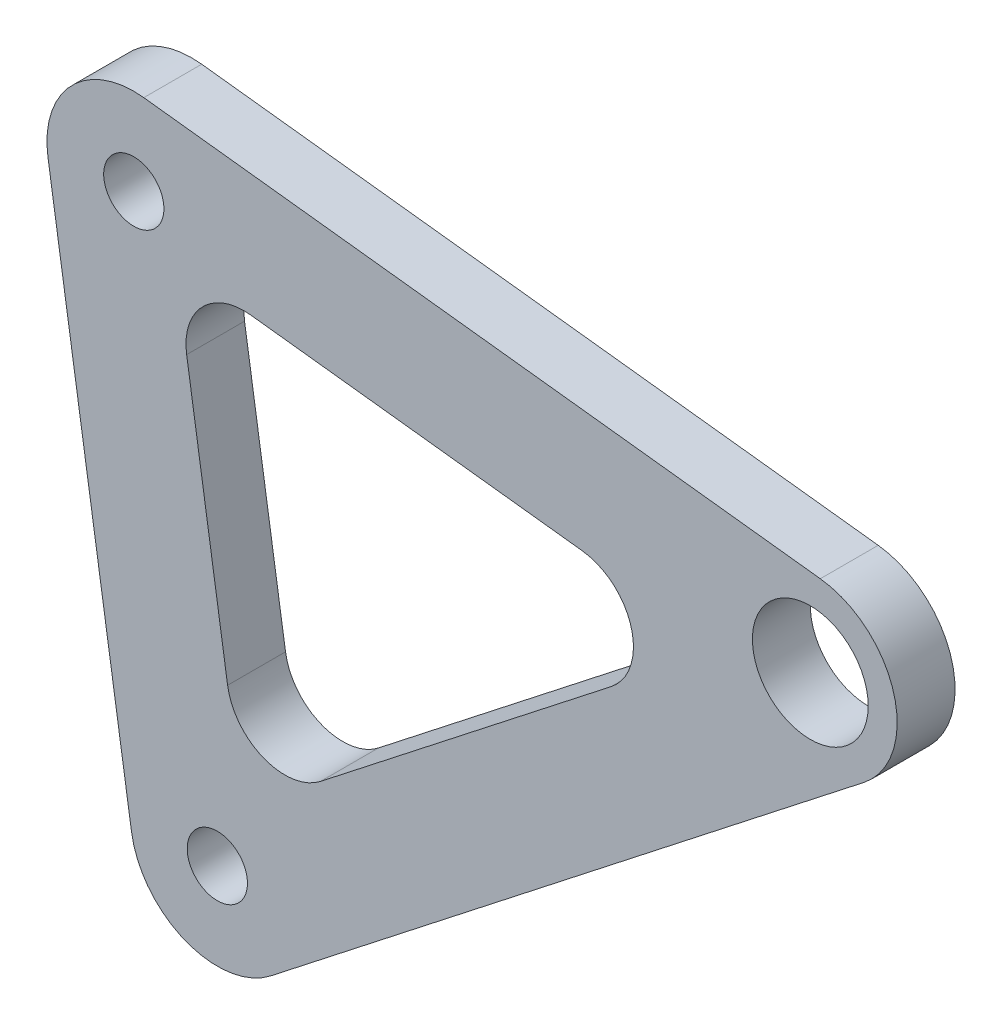
SolidWorks part; units mm, degrees
ref_plane "Front Plane" through (0, 0, 0) normal (0, 0, 1) x (1, 0, 0)
ref_plane "Top Plane" through (0, 0, 0) normal (0, 1, 0) x (1, 0, 0)
ref_plane "Right Plane" through (0, 0, 0) normal (1, 0, 0) x (0, 0, -1)
other "Configuration Table"
sketch "Sketch1" plane through (0, 0, 0) normal (0, 0, 1) x (1, 0, 0)
  line L0 (7.214, -46.8294) -> (58.4141, -6.7676) construction
  line L1 (58.4141, -6.7676) -> (0, 0) construction
  line L2 (0, 0) -> (7.214, -46.8294) construction
  line L3 (-7.4126, -1.1419) -> (-0.1986, -47.9713)
  line L4 (11.8357, -52.7362) -> (63.0359, -12.6743)
  line L5 (59.2773, 0.6826) -> (0.8631, 7.4502)
  line L6 (38.7166, -7.5056) -> (10.0801, -4.1879)
  line L7 (4.5629, -9.9159) -> (8.0995, -32.8733)
  line L8 (16.1223, -36.0498) -> (41.2224, -16.4102)
  line L9 (9.3992, -41.3104) -> (50.8118, -8.9069) construction
  line L10 (1.751, -60.627) -> (77.42, -1.4193) construction
  line L11 (77.42, -1.4193) -> (-8.9106, 8.5825) construction
  line L12 (-8.9106, 8.5825) -> (1.751, -60.627) construction
  line L13 (3.5642, -3.433) -> (9.3992, -41.3104) construction
  line L14 (50.8118, -8.9069) -> (3.5642, -3.433) construction
  circle A0 centre (58.4141, -6.7676) radius 5
  circle A1 centre (7.214, -46.8294) radius 2.6
  circle A2 centre (0, 0) radius 2.6
  arc A3 (0.8631, 7.4502) -> (-7.4126, -1.1419) centre (0, 0) ccw
  arc A4 (63.0359, -12.6743) -> (59.2773, 0.6826) centre (58.4141, -6.7676) ccw
  arc A5 (-0.1986, -47.9713) -> (11.8357, -52.7362) centre (7.214, -46.8294) ccw
  arc A6 (16.1223, -36.0498) -> (8.0995, -32.8733) centre (13.0412, -32.112) cw
  arc A7 (41.2224, -16.4102) -> (38.7166, -7.5056) centre (38.1412, -12.4724) ccw
  arc A8 (4.5629, -9.9159) -> (10.0801, -4.1879) centre (9.5046, -9.1547) cw
  dimension "D5" = 5.2
  dimension "D6" = 15
  dimension "D9" = 5
  dimension "D10" = 10
  dimension "D1" = 46.8294
  dimension "D2" = 7.214
  dimension "D3" = 6.7676
  dimension "D4" = 58.4141
  dimension "D7" = 7.5
  dimension "D8" = 3
extrude "Boss-Extrude1" add sketch "Sketch1" along normal blind 5
